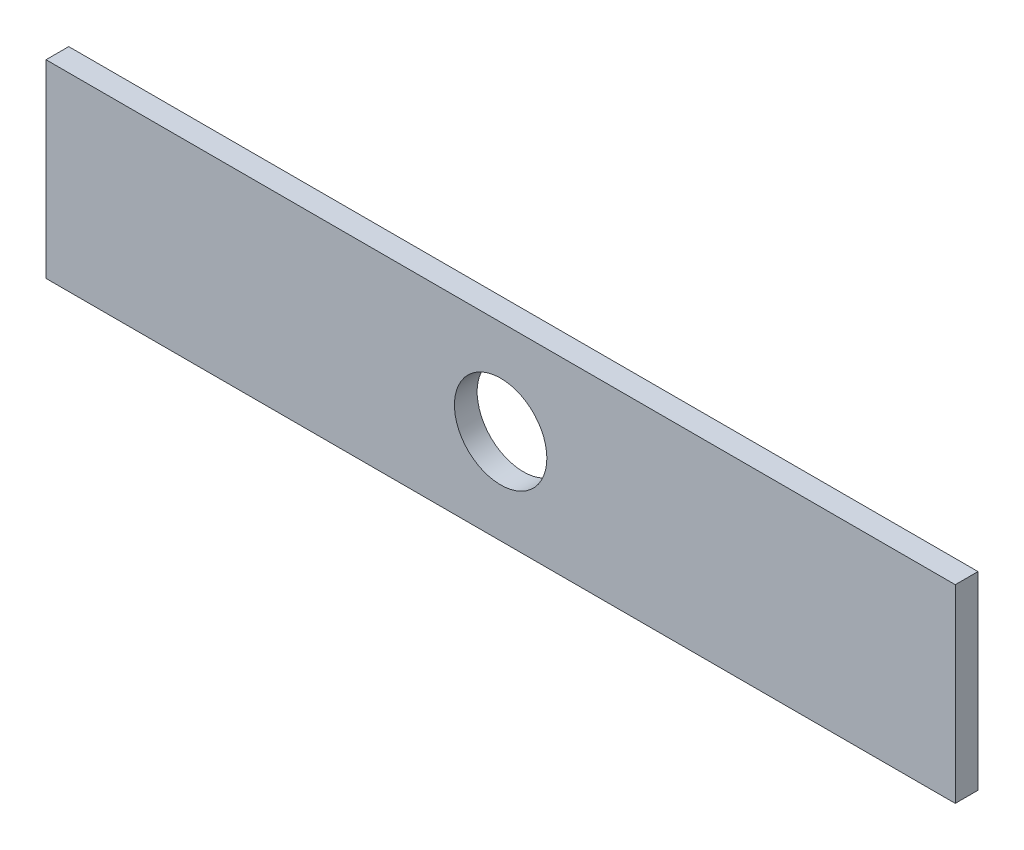
SolidWorks part; units mm, degrees
ref_plane "前视基准面" through (0, 0, 0) normal (0, 0, 1) x (1, 0, 0)
ref_plane "上视基准面" through (0, 0, 0) normal (0, 1, 0) x (1, 0, 0)
ref_plane "右视基准面" through (0, 0, 0) normal (1, 0, 0) x (0, 0, -1)
other "Configuration Table"
sketch "草图1" plane through (0, 0, 0) normal (0, 0, 1) x (1, 0, 0)
  line L0 (-60, -12.5) -> (60, -12.5)
  line L1 (60, -12.5) -> (60, 12.5)
  line L2 (60, 12.5) -> (-60, 12.5)
  line L3 (-60, 12.5) -> (-60, -12.5)
  point P0 (0, 0)
  dimension "D1" = 60
  dimension "D2" = 120
  dimension "D3" = 12.5
  dimension "D4" = 25
extrude "凸台-拉伸1" add sketch "草图1" against normal mid plane 3
sketch "草图2" plane through (0, 0, 0) normal (0, 0, 1) x (1, 0, 0)
  circle A0 centre (0, 0) radius 6.1
  point P0 (0, 0)
  dimension "D1" = 12.2
extrude "切除-拉伸1" cut sketch "草图2" against normal mid plane 23
